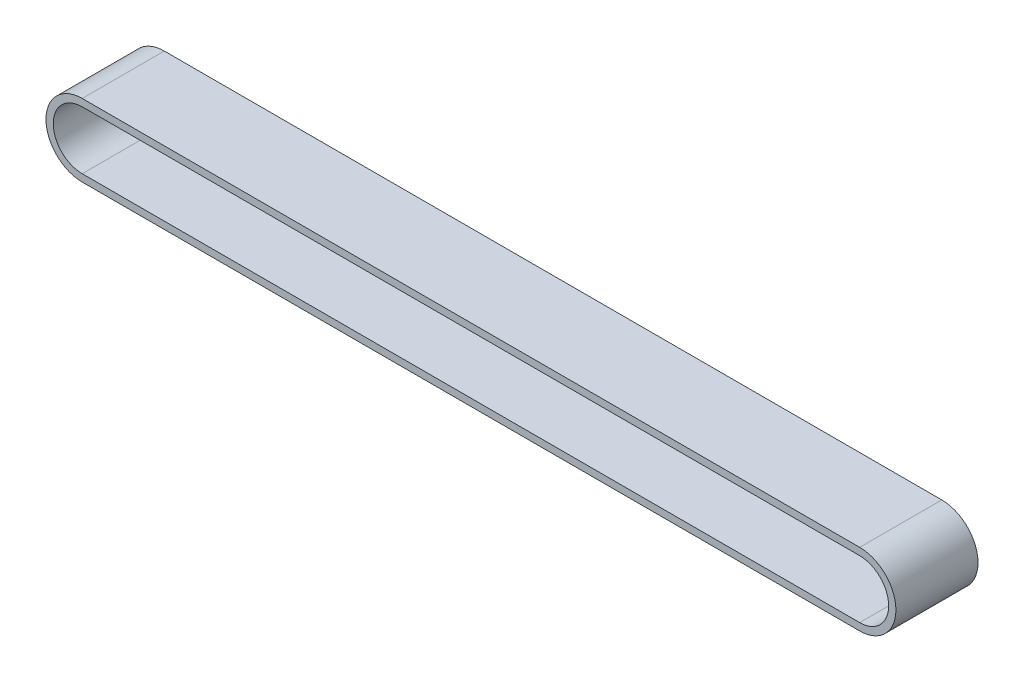
SolidWorks part; units mm, degrees
ref_plane "前视基准面" through (0, 0, 0) normal (0, 0, 1) x (1, 0, 0)
ref_plane "上视基准面" through (0, 0, 0) normal (0, 1, 0) x (1, 0, 0)
ref_plane "右视基准面" through (0, 0, 0) normal (1, 0, 0) x (0, 0, -1)
other "Configuration Table"
sketch "草图1" plane through (0, 0, 0) normal (0, 0, 1) x (1, 0, 0)
  line L0 (0, 60) -> (-1610, 60)
  line L1 (0, -60) -> (-1610, -60)
  line L2 (0, 75) -> (-1610, 75)
  line L3 (0, -75) -> (-1610, -75)
  arc A0 (0, -60) -> (0, 60) centre (0, 0) ccw
  arc A1 (-1610, 60) -> (-1610, -60) centre (-1610, 0) ccw
  arc A2 (-1610, 75) -> (-1610, -75) centre (-1610, 0) ccw
  arc A3 (0, -75) -> (0, 75) centre (0, 0) ccw
  dimension "D1" = 60
  dimension "D2" = 60
  dimension "D4" = 60
  dimension "D3" = 1610
  dimension "D5" = 15
extrude "凸台-拉伸1" add sketch "草图1" along normal blind 170
